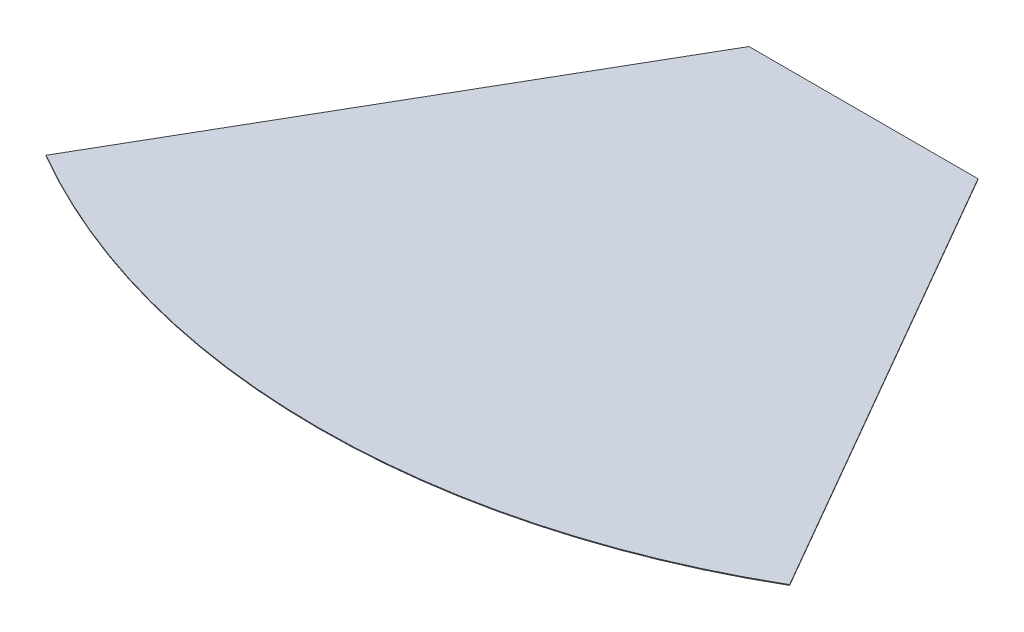
from build123d import *

# Parameters (mm, degrees)
BOSS_EXTRUDE1_DEPTH = 3


with BuildPart() as part:
    # Sketch1 → Boss-Extrude1 (new body)
    with BuildSketch(Plane(origin=(0, 0, 0), x_dir=(1, 0, 0), z_dir=(0, 1, 0))):
        with BuildLine():
            Line((-462, 0), (462, 0))
            Line((462, 0), (1500, -1797.868738256))
            ThreePointArc((1500, -1797.868738256), (0, -2199.792526903), (-1500, -1797.868738256))
            Line((-1500, -1797.868738256), (-462, 0))
        make_face()
    extrude(amount=BOSS_EXTRUDE1_DEPTH)


solid = part.part
